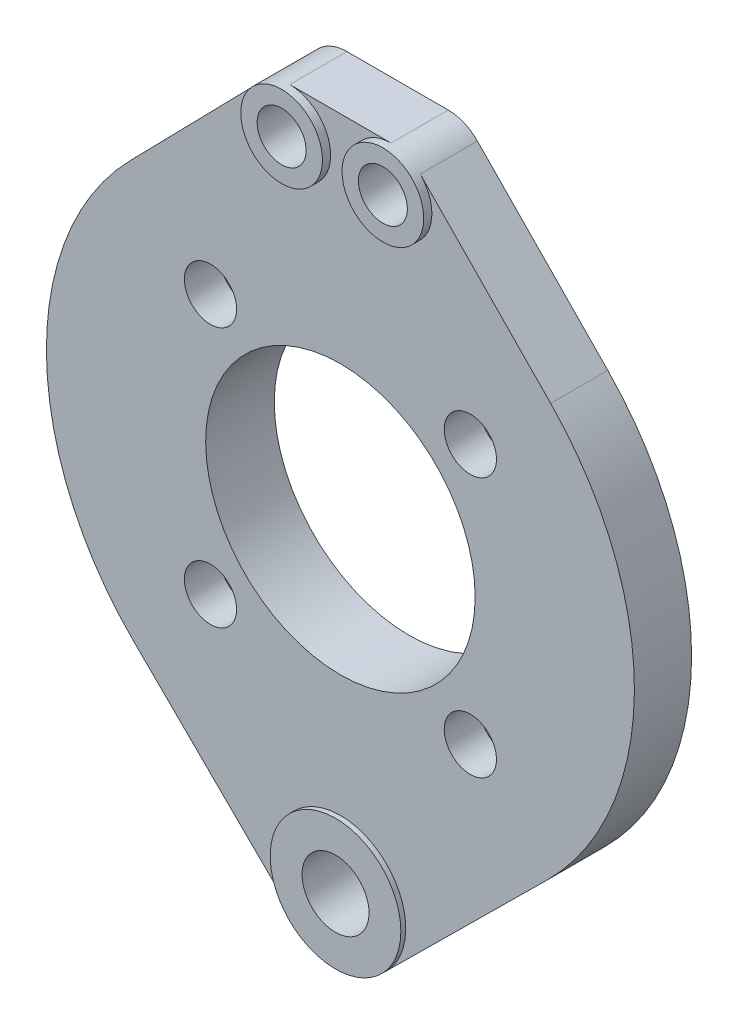
from build123d import *
from build123d.topology import SkipClean

# Parameters (mm, degrees)
SKETCH1_R          = 15
SKETCH1_R_2        = 20.5
SKETCH1_R_3        = 82.5
EXTRUDE1_DEPTH     = 35
SKETCH2_R          = 25
SKETCH2_R_2        = 15
EXTRUDE2_DEPTH     = 5
CUT_EXTRUDE1_REACH = 301.656
SKETCH3_R          = 11
SKETCH5_R          = 16
CUT_EXTRUDE9_DEPTH = 22
CIRPATTERN1_COUNT  = 4
SKETCH8_R          = 40
SKETCH8_R_2        = 20.5
EXTRUDE5_DEPTH     = 3
EXTRUDE6_START     = 7
SKETCH9_R          = 90
SKETCH9_R_2        = 82.5
EXTRUDE6_DEPTH     = 7


with BuildPart() as part:
    # Sketch1 → Extrude1 (new body)
    with BuildSketch(Plane.XY):
        with BuildLine():
            Line((-48.874792723, 207.478323293), (-128.698507603, 125.843927707))
            ThreePointArc((-128.698507603, 125.843927707), (-179.994057412, -1.462633346), (-126.636429521, -127.918781726))
            Line((-126.636429521, -127.918781726), (-28.141428782, -225.426395939))
            ThreePointArc((-28.141428782, -225.426395939), (0, -237), (28.141428782, -225.426395939))
            Line((28.141428782, -225.426395939), (126.636429521, -127.918781726))
            ThreePointArc((126.636429521, -127.918781726), (179.994057412, -1.462633346), (128.698507603, 125.843927707))
            Line((128.698507603, 125.843927707), (48.874792723, 207.478323293))
            ThreePointArc((48.874792723, 207.478323293), (40.696440524, 213.042982471), (31, 215))
            Line((31, 215), (-31, 215))
            ThreePointArc((-31, 215), (-40.696440524, 213.042982471), (-48.874792723, 207.478323293))
        make_face()
        with Locations((-31, 190)):
            Circle(SKETCH1_R, mode=Mode.SUBTRACT)
        with Locations((31, 190)):
            Circle(SKETCH1_R, mode=Mode.SUBTRACT)
        with Locations((0, -197)):
            Circle(SKETCH1_R_2, mode=Mode.SUBTRACT)
        Circle(SKETCH1_R_3, mode=Mode.SUBTRACT)
    extrude(amount=EXTRUDE1_DEPTH)

    # Sketch2 → Extrude2 (add)
    # profile 1 of 2: a face of its own
    with BuildSketch(Plane.XY.offset(35)):
        with Locations(Location((-31, 190, 0), (0, 0, 135.642519681))):
            Circle(SKETCH2_R)
        with Locations((-31, 190)):
            Circle(SKETCH2_R_2, mode=Mode.SUBTRACT)
    # profile 2 of 2: a face of its own
    with BuildSketch(Plane.XY.offset(35)):
        with Locations(Location((31, 190, 0), (0, 0, 90))):
            Circle(SKETCH2_R)
        with Locations((31, 190)):
            Circle(SKETCH2_R_2, mode=Mode.SUBTRACT)
    extrude(amount=EXTRUDE2_DEPTH)

    # Sketch3 → Cut-Extrude1 (cut, up to next)
    with BuildSketch(Plane.XY.offset(35), mode=Mode.PRIVATE) as cut_extrude1_sk1:
        with Locations((-79.549512883, 79.549512883)):
            Circle(SKETCH3_R)
    cut_extrude1_tool1 = extrude(cut_extrude1_sk1.sketch, amount=-CUT_EXTRUDE1_REACH, mode=Mode.PRIVATE) & part.part
    # Sketch3 → Cut-Extrude1 (cut, up to next)
    with BuildSketch(Plane.XY.offset(35), mode=Mode.PRIVATE) as cut_extrude1_sk2:
        with Locations((-79.549512883, -79.549512883)):
            Circle(SKETCH3_R)
    cut_extrude1_tool2 = extrude(cut_extrude1_sk2.sketch, amount=-CUT_EXTRUDE1_REACH, mode=Mode.PRIVATE) & part.part
    # Sketch3 → Cut-Extrude1 (cut, up to next)
    with BuildSketch(Plane.XY.offset(35), mode=Mode.PRIVATE) as cut_extrude1_sk3:
        with Locations((79.549512883, -79.549512883)):
            Circle(SKETCH3_R)
    cut_extrude1_tool3 = extrude(cut_extrude1_sk3.sketch, amount=-CUT_EXTRUDE1_REACH, mode=Mode.PRIVATE) & part.part
    # Sketch3 → Cut-Extrude1 (cut, up to next)
    with BuildSketch(Plane.XY.offset(35), mode=Mode.PRIVATE) as cut_extrude1_sk4:
        with Locations((79.549512883, 79.549512883)):
            Circle(SKETCH3_R)
    cut_extrude1_tool4 = extrude(cut_extrude1_sk4.sketch, amount=-CUT_EXTRUDE1_REACH, mode=Mode.PRIVATE) & part.part
    add(cut_extrude1_tool1.solids().sort_by_distance((-79.549513, 79.549513, 35))[0], mode=Mode.SUBTRACT)
    add(cut_extrude1_tool2.solids().sort_by_distance((-79.549513, -79.549513, 35))[0], mode=Mode.SUBTRACT)
    add(cut_extrude1_tool3.solids().sort_by_distance((79.549513, -79.549513, 35))[0], mode=Mode.SUBTRACT)
    add(cut_extrude1_tool4.solids().sort_by_distance((79.549513, 79.549513, 35))[0], mode=Mode.SUBTRACT)

    # Sketch5 → Cut-Extrude9 (cut)
    with BuildSketch(Plane.XY.offset(35)):
        with Locations((-79.549512883, 79.549512883)):
            Circle(SKETCH5_R)
    cut_extrude9 = extrude(amount=-CUT_EXTRUDE9_DEPTH, mode=Mode.SUBTRACT)

    # CirPattern1: Cut-Extrude9 ×4 about axis
    cirpattern1_axis = Axis((0, 0, 0), (0, 0, 1))
    for i in range(1, CIRPATTERN1_COUNT):
        add(cut_extrude9.rotate(cirpattern1_axis, i * 360 / CIRPATTERN1_COUNT), mode=Mode.SUBTRACT)

    # Sketch8 → Extrude5 (add)
    with BuildSketch(Plane.XY.offset(35)):
        with Locations(Location((0, -197, 0), (0, 0, 225.288631874))):
            Circle(SKETCH8_R)
        with Locations((0, -197)):
            Circle(SKETCH8_R_2, mode=Mode.SUBTRACT)
    extrude(amount=EXTRUDE5_DEPTH)

    # Sketch9 → Extrude6 (add)
    with SkipClean():  # the faces are left unmerged after this step: merging them gives an invalid solid
        with BuildSketch(Plane(origin=(0, 0, 0), x_dir=(-1, 0, 0), z_dir=(0, 0, -1)).offset(EXTRUDE6_START)):
            with Locations(Location((0, 0, 0), (0, 0, 180))):
                Circle(SKETCH9_R)
            Circle(SKETCH9_R_2, mode=Mode.SUBTRACT)
        extrude(amount=-EXTRUDE6_DEPTH)


solid = part.part
